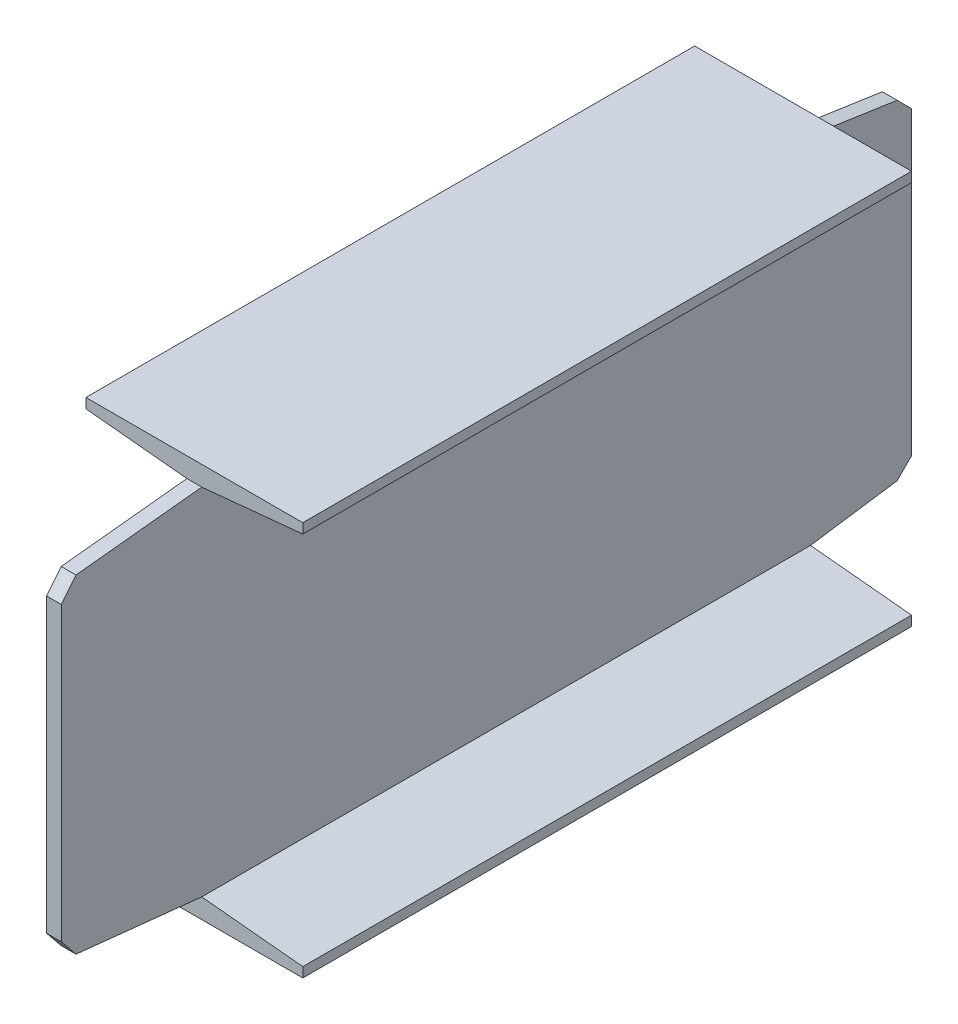
from build123d import *
from OCP.BRepFilletAPI import BRepFilletAPI_MakeChamfer

# Parameters (mm, degrees)
EXTRUDE_1_DEPTH          = 172.5
CUT_EXTRUDE_1_DEPTH      = 196.172359723
CUT_EXTRUDE_1_DEPTH_BACK = 196.172359723
CHAMFER_1_SIZE           = 6
CHAMFER_1_SIZE2          = 6.742931709
CHAMFER_2_SIZE           = 5
CHAMFER_2_SIZE2          = 5.919528387
CHAMFER_2_EDGE_2_SIZE    = 5
CHAMFER_2_EDGE_2_SIZE2   = 5.919528387


with BuildPart() as part:
    # 草图1 → 凸台-拉伸1 (new, symmetric)
    with BuildSketch(Plane.XY):
        Polygon((44, 80), (-44, 80), (-44, 76), (-3, 72), (-3, -72), (-44, -76), (-44, -80), (44, -80), (44, -76), (3, -72), (3, 72), (44, 76), align=None)
    extrude(amount=EXTRUDE_1_DEPTH, both=True)

    # 草图3 → 切除-拉伸1 (cut, two sides: drawn at the far end of the back side and taken through both)
    with BuildSketch(Plane(origin=(0, 0, 0), x_dir=(0, 0, -1), z_dir=(1, 0, 0)).offset(-CUT_EXTRUDE_1_DEPTH_BACK)):
        Polygon((-172.5, 66), (-115.5, 72), (-115.5, 80), (-172.5, 80), align=None)
        Polygon((172.5, 80), (172.5, 66), (131.5, 72), (131.5, 80), align=None)
        Polygon((172.5, -66), (131.5, -72), (131.5, -80), (172.5, -80), align=None)
        Polygon((-172.5, -80), (-172.5, -66), (-115.5, -72), (-115.5, -80), align=None)
    extrude(amount=CUT_EXTRUDE_1_DEPTH + CUT_EXTRUDE_1_DEPTH_BACK, mode=Mode.SUBTRACT)

    # 倒角1: one chamfer whose edges measure the first distance from different faces: ONE call of the kernel's chamfer builder (chamfer() names one face for all edges)
    chamfer_1_edges_1 = [part.edges().sort_by_distance(p)[0] for p in [
        (0, 66, 172.5),
    ]]
    chamfer_1_side_1 = [part.faces().sort_by_distance(p)[0] for p in [
        (0, 69, 144),
    ]]
    chamfer_1_edges_2 = [part.edges().sort_by_distance(p)[0] for p in [
        (0, -66, 172.5),
    ]]
    chamfer_1_side_2 = [part.faces().sort_by_distance(p)[0] for p in [
        (0, -69, 144),
    ]]
    chamfer_1 = BRepFilletAPI_MakeChamfer(part.part.solid().wrapped)
    for e in chamfer_1_edges_1:
        chamfer_1.Add(CHAMFER_1_SIZE, CHAMFER_1_SIZE2, e.wrapped, chamfer_1_side_1[0].wrapped)  # the first distance lies on this face
    for e in chamfer_1_edges_2:
        chamfer_1.Add(CHAMFER_1_SIZE, CHAMFER_1_SIZE2, e.wrapped, chamfer_1_side_2[0].wrapped)  # the first distance lies on this face
    add(Compound.cast(chamfer_1.Shape()), mode=Mode.REPLACE)

    # 倒角2
    chamfer_2_edges = [part.edges().sort_by_distance(p)[0] for p in [
        (0, 66, -172.5),
    ]]
    chamfer_2_side = [part.faces().sort_by_distance(p)[0] for p in [
        (0, 0, -172.5),
    ]]
    chamfer(chamfer_2_edges, length=CHAMFER_2_SIZE, length2=CHAMFER_2_SIZE2, reference=chamfer_2_side[0])

    # 倒角2 edge 2
    chamfer_2_edge_2_edges = [part.edges().sort_by_distance(p)[0] for p in [
        (0, -66, -172.5),
    ]]
    chamfer_2_edge_2_side = [part.faces().sort_by_distance(p)[0] for p in [
        (0, 0, -172.5),
    ]]
    chamfer(chamfer_2_edge_2_edges, length=CHAMFER_2_EDGE_2_SIZE, length2=CHAMFER_2_EDGE_2_SIZE2, reference=chamfer_2_edge_2_side[0])


solid = part.part
